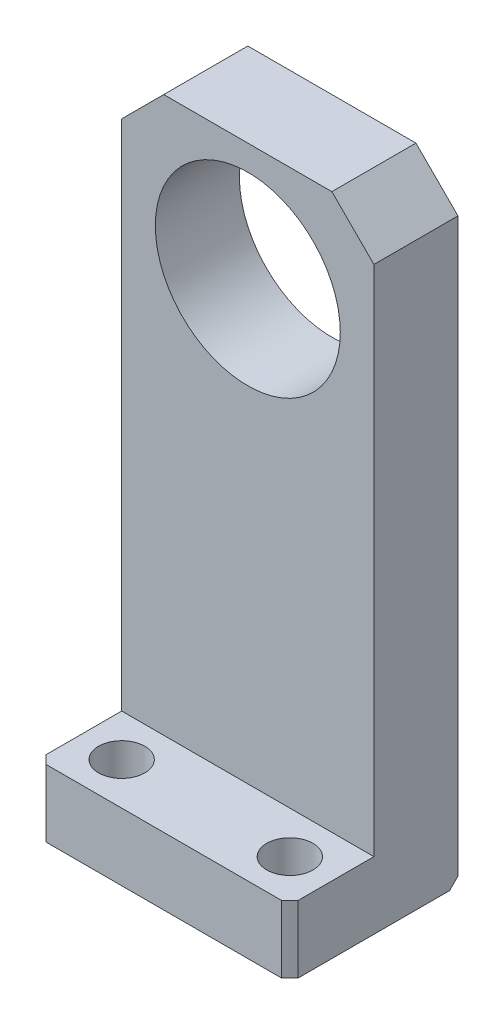
from build123d import *

# Parameters (mm, degrees)
SKETCH1_W                    = 30
SKETCH1_H                    = 74
SKETCH1_R                    = 11
BOSS_EXTRUDE1_DEPTH          = 10
SKETCH3_W                    = 15
SKETCH3_H                    = 10
BOSS_EXTRUDE2_DEPTH          = 8
SKETCH4_R                    = 2.75
CUT_EXTRUDE1_DEPTH           = 71.576199954
F_4_0_4_DIAMETER_HOLE1_D     = 4
F_4_0_4_DIAMETER_HOLE1_DEPTH = 10
F_4_0_4_DIAMETER_HOLE1_TIP   = 1.201721238
CHAMFER1_SIZE                = 5
CHAMFER2_SIZE                = 1


with BuildPart() as part:
    # Sketch1 → Boss-Extrude1 (new body)
    with BuildSketch(Plane.XY):
        with Locations((0, 37)):
            Rectangle(SKETCH1_W, SKETCH1_H)
        with Locations((0, 60)):
            Circle(SKETCH1_R, mode=Mode.SUBTRACT)
    extrude(amount=BOSS_EXTRUDE1_DEPTH)

    # Sketch3 → Boss-Extrude2 (add)
    with BuildSketch(Plane.XZ):
        with Locations((-7.5, 15)):
            Rectangle(SKETCH3_W, SKETCH3_H)
        with Locations((7.5, 15)):
            Rectangle(SKETCH3_W, SKETCH3_H)
    extrude(amount=-BOSS_EXTRUDE2_DEPTH)

    # Sketch4 → Cut-Extrude1 (cut, through all)
    with BuildSketch(Plane(origin=(0, 8, 0), x_dir=(-1, 0, 0), z_dir=(0, 1, 0))):
        with Locations((10, 15)):
            Circle(SKETCH4_R)
        with Locations(Location((-10, 15, 0), (0, 0, 180))):
            Circle(SKETCH4_R)
    extrude(amount=-CUT_EXTRUDE1_DEPTH, mode=Mode.SUBTRACT)

    # Ø4.0 (4) Diameter Hole1
    with Locations(Plane.XZ):
        with Locations((-10, 5), (10, 5)):
            Hole(F_4_0_4_DIAMETER_HOLE1_D / 2, depth=F_4_0_4_DIAMETER_HOLE1_DEPTH)
            with Locations((0, 0, -(F_4_0_4_DIAMETER_HOLE1_DEPTH + F_4_0_4_DIAMETER_HOLE1_TIP / 2))):  # 118° drill point
                Cone(0, F_4_0_4_DIAMETER_HOLE1_D / 2, F_4_0_4_DIAMETER_HOLE1_TIP, mode=Mode.SUBTRACT)

    # Chamfer1
    chamfer1_edges = [part.edges().sort_by_distance(p)[0] for p in [
        (-15, 74, 5),
        (15, 74, 5),
    ]]
    chamfer(chamfer1_edges, length=CHAMFER1_SIZE)

    # Chamfer2
    chamfer2_edges = [part.edges().sort_by_distance(p)[0] for p in [
        (-15, 4, 20),
        (15, 4, 20),
        (0, 0, 0),
    ]]
    chamfer(chamfer2_edges, length=CHAMFER2_SIZE)


solid = part.part
